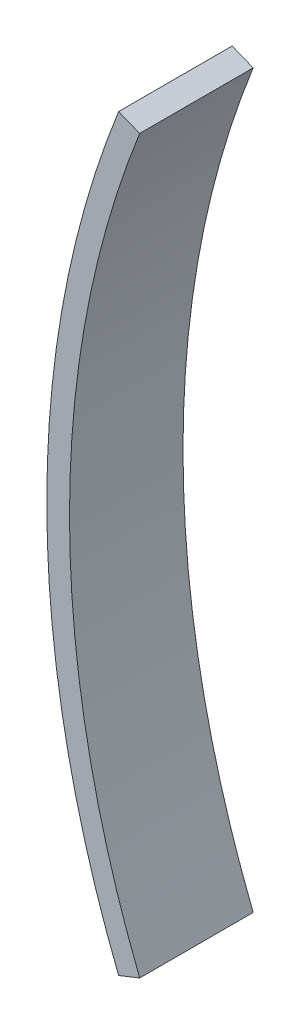
from build123d import *

# Parameters (mm, degrees)
BOSS_EXTRUDE1_DEPTH = 31.75


with BuildPart() as part:
    # Sketch1 → Boss-Extrude1 (new body)
    with BuildSketch(Plane.XY):
        with BuildLine():
            Line((-256.713821989, 102.31), (-262.61261978, 104.660890176))
            ThreePointArc((-262.61261978, 104.660890176), (-282.7, 0), (-262.61261978, -104.660890176))
            Line((-262.61261978, -104.660890176), (-256.713821989, -102.31))
            ThreePointArc((-256.713821989, -102.31), (-276.35, 0), (-256.713821989, 102.31))
        make_face()
    extrude(amount=BOSS_EXTRUDE1_DEPTH)


solid = part.part
